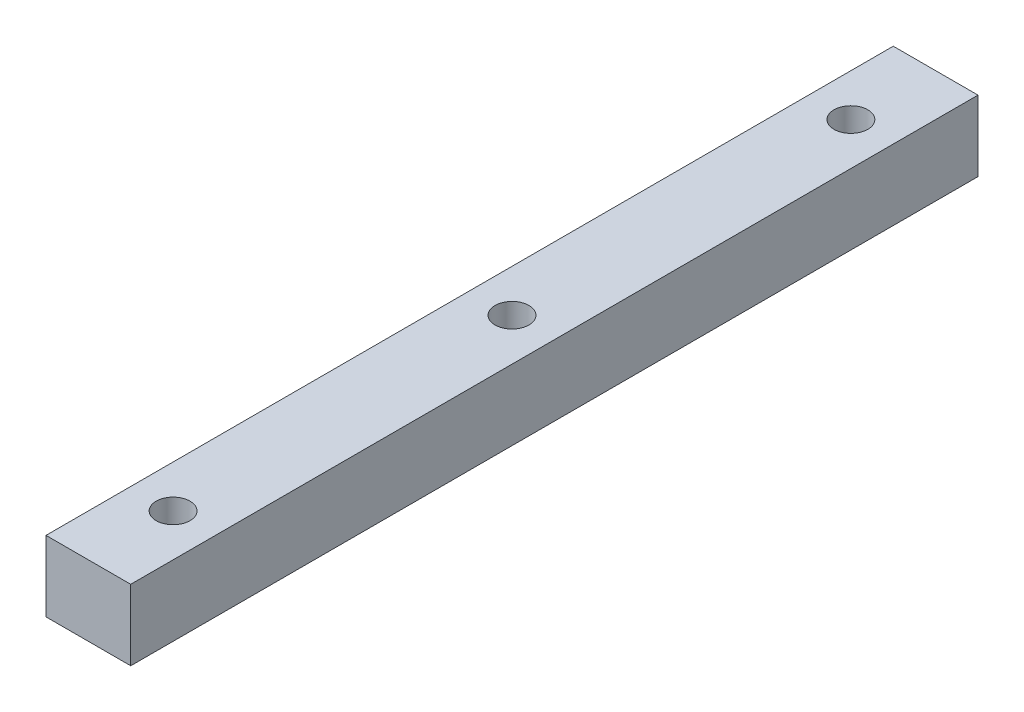
from build123d import *

# Parameters (mm, degrees)
SKETCH_1_W             = 15
SKETCH_1_H             = 12.5
EXTRUDE_1_DEPTH        = 75
SKETCH_2_R             = 3
CUT_EXTRUDE_1_DEPTH    = 4.5
SKETCH_3_R             = 2
CUT_EXTRUDE_2_DEPTH    = 77.40353395
PATTERN_LINEAR_1_COUNT = 6
PATTERN_LINEAR_1_PITCH = 60


with BuildPart() as part:
    # 草图1 → 凸台-拉伸1 (new, symmetric)
    with BuildSketch(Plane.XY):
        Rectangle(SKETCH_1_W, SKETCH_1_H)
    extrude(amount=EXTRUDE_1_DEPTH, both=True)

    # 草图2 → 切除-拉伸1 (cut)
    with BuildSketch(Plane(origin=(0, 6.25, 0), x_dir=(1, 0, 0), z_dir=(0, 1, 0))):
        with Locations(Location((0, -60, 0), (0, 0, 270))):
            Circle(SKETCH_2_R)
    cut_extrude_1 = extrude(amount=-CUT_EXTRUDE_1_DEPTH, mode=Mode.SUBTRACT)

    # 草图3 → 切除-拉伸2 (cut, through all)
    with BuildSketch(Plane(origin=(0, 6.25, 0), x_dir=(1, 0, 0), z_dir=(0, 1, 0))):
        with Locations(Location((0, -60, 0), (0, 0, 270))):
            Circle(SKETCH_3_R)
    cut_extrude_2 = extrude(amount=-CUT_EXTRUDE_2_DEPTH, mode=Mode.SUBTRACT)

    # 阵列(线性)1: 切除-拉伸1, 切除-拉伸2 ×6
    with Locations(*[(0, 0, -i * PATTERN_LINEAR_1_PITCH) for i in range(1, PATTERN_LINEAR_1_COUNT)]):
        add(cut_extrude_1, mode=Mode.SUBTRACT)
        add(cut_extrude_2, mode=Mode.SUBTRACT)


solid = part.part
